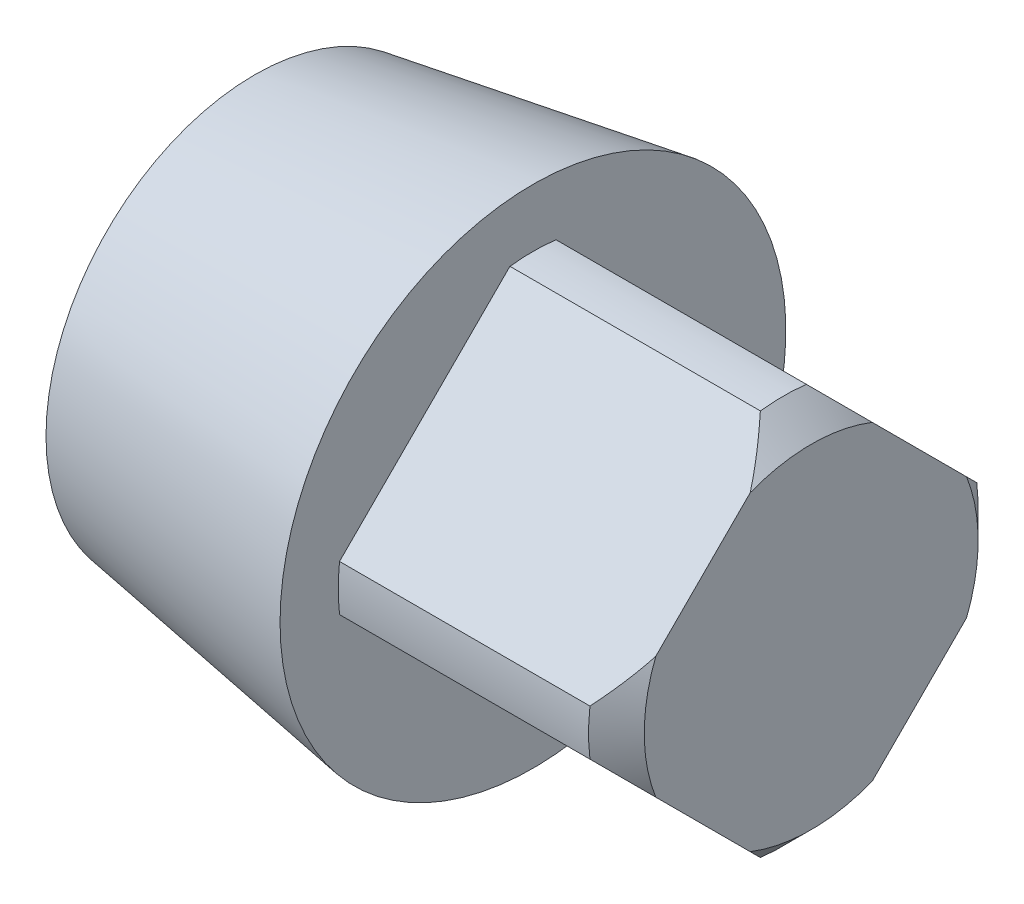
SolidWorks part; units mm, degrees
ref_plane "Front Plane" through (0, 0, 0) normal (0, 0, 1) x (1, 0, 0)
ref_plane "Top Plane" through (0, 0, 0) normal (0, 1, 0) x (1, 0, 0)
ref_plane "Right Plane" through (0, 0, 0) normal (1, 0, 0) x (0, 0, -1)
sketch "Sketch1" plane through (0, 0, 0) normal (0, 0, 1) x (1, 0, 0)
  line L0 (10.16, 16.614) -> (10.16, 0) construction
  line L9 (0, 0) -> (20, 0)
  line L10 (0, 0) -> (0, 15)
  line L11 (0, 15) -> (20, 18.1772)
  line L12 (20, 14) -> (20, 18.1772)
  line L13 (20, 0) -> (40, 0)
  line L14 (20, 0) -> (20, 14) construction
  line L15 (20, 14) -> (40, 14)
  line L16 (40, 0) -> (40, 14)
  line L17 (20, 0) -> (20, 14) construction
  dimension "D1" = 20
  dimension "D2" = 14
  dimension "D3" = 20
  dimension "D4" = 10.16
  dimension "D5" = 16.614
  dimension "D6" = 15
revolve "Revolve1" add sketch "Sketch1" angle 360 about L13
chamfer "Chamfer1" distance 2 angle 45 1 edges at (40, 0, 14)
sketch "Sketch2" plane through (40, 0, 0) normal (1, 0, 0) x (0, 0, -1)
  line L0 (0, 0) -> (0, -15.5563) construction
  line L1 (0, -15.5563) -> (15.5563, 0)
  line L2 (15.5563, 0) -> (0, 15.5563)
  line L3 (0, 15.5563) -> (-15.5563, 0)
  line L4 (-15.5563, 0) -> (0, -15.5563)
  circle A0 centre (0, 0) radius 11 construction
  circle A1 centre (0, 0) radius 14 construction
  circle A2 centre (0, 0) radius 14
  circle M1 centre (0, 0) radius 12
  dimension "D1" = 22
extrude "Cut-Extrude1" cut sketch "Sketch2" against normal blind 20 contours L2 A2 M1 | L2 M1
pattern_circular "CirPattern1" count 4 over 360 about axis through (0, 0, 0) along (1, 0, 0) of "Cut-Extrude1"
